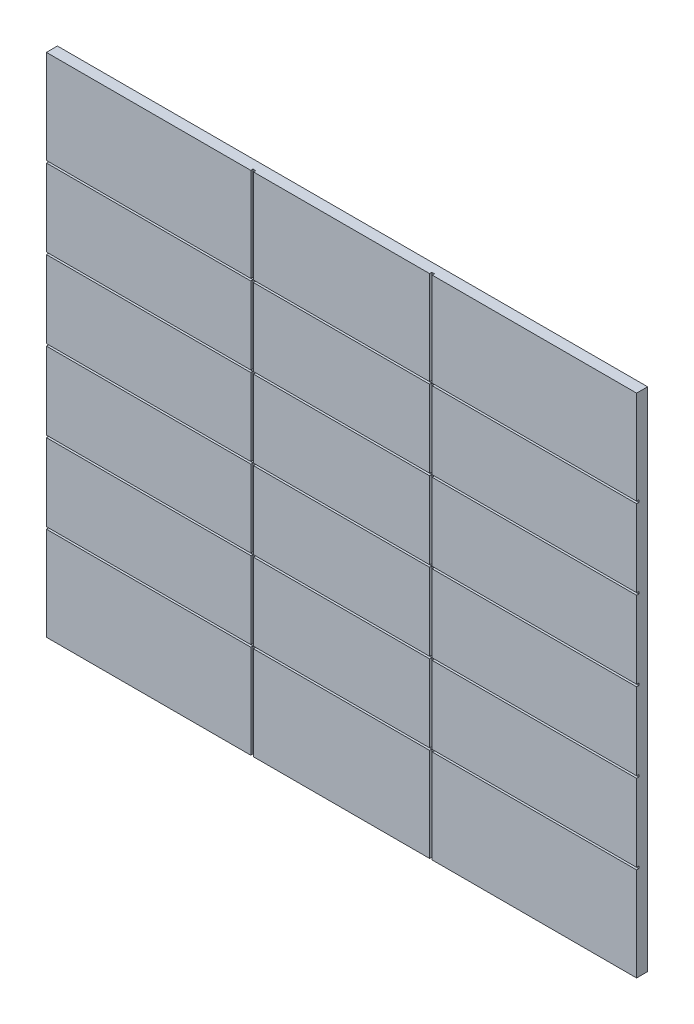
SolidWorks part; units mm, degrees
ref_plane "Front Plane" through (0, 0, 0) normal (0, 0, 1) x (1, 0, 0)
ref_plane "Top Plane" through (0, 0, 0) normal (0, 1, 0) x (1, 0, 0)
ref_plane "Right Plane" through (0, 0, 0) normal (1, 0, 0) x (0, 0, -1)
sketch "Sketch1" plane through (0, 0, 0) normal (0, 0, 1) x (1, 0, 0)
  line L1 (-670, 575) -> (670, 575)
  line L2 (-670, 575) -> (-670, -575)
  line L3 (-670, -575) -> (670, -575)
  line L4 (670, 575) -> (670, -575)
  line L5 (-670, 575) -> (670, -575) construction
  line L6 (-670, -575) -> (670, 575) construction
  point P0 (0, 0)
  dimension "D1" = 1340
  dimension "D2" = 1150
extrude "Boss-Extrude1" add sketch "Sketch1" along normal blind 25
sketch "Sketch2" plane through (0, 0, 25) normal (0, 0, 1) x (1, 0, 0)
  line L1 (-689.8522, 2.5) -> (689.8522, 2.5)
  line L2 (-689.8522, 2.5) -> (-689.8522, -2.5)
  line L3 (-689.8522, -2.5) -> (689.8522, -2.5)
  line L4 (689.8522, 2.5) -> (689.8522, -2.5)
  line L5 (-689.8522, 2.5) -> (689.8522, -2.5) construction
  line L6 (-689.8522, -2.5) -> (689.8522, 2.5) construction
  point P0 (0, 0)
  dimension "D1" = 5
extrude "Cut-Extrude1" cut sketch "Sketch2" against normal blind 5
sketch "Sketch3" plane through (0, 0, 25) normal (0, 0, 1) x (1, 0, 0)
  line L0 (0, 0) -> (0, 486.5607) construction
  line L1 (200, 577.0918) -> (206, 577.0918)
  line L2 (200, 577.0918) -> (200, -578.2429)
  line L3 (200, -578.2429) -> (206, -578.2429)
  line L4 (206, 577.0918) -> (206, -578.2429)
  line L5 (200, 577.0918) -> (206, -578.2429) construction
  line L6 (200, -578.2429) -> (206, 577.0918) construction
  line L7 (-200, 577.0918) -> (-206, 577.0918)
  line L8 (-200, -578.2429) -> (-206, -578.2429)
  line L9 (-206, 577.0918) -> (-206, -578.2429)
  line L10 (-200, 577.0918) -> (-200, -578.2429)
  point P0 (203, -0.5755)
  dimension "D1" = 6
  dimension "D2" = 200
extrude "Cut-Extrude2" cut sketch "Sketch3" against normal blind 5
pattern_linear "LPattern1" count 3 spacing 180 along (0, -1, 0) count 3 spacing 180 along (0, 1, 0) seed only of "Cut-Extrude1"
sketch "Sketch4" plane through (-49.5237, -434, -370.2813) normal (0, -1, 0) x (0.9899, 0, -0.1414)
  line L0 (362.9416, 425.8894) -> (367.1842, 396.1909)
  line L1 (-666.6059, 278.8112) -> (659.9264, 468.3158) construction
  line L2 (656.3909, 493.0646) -> (659.9264, 468.3158) construction
  dimension "D1" = 30
  dimension "D2" = 300
sweep "Sweep1" add path "Sketch4" circular profile diameter 10 parameters "D3"=10
sketch "Sketch13" plane through (0, 0, -30) normal (0, 0, -1) x (-1, 0, 0)
  circle A0 centre (-370, -434) radius 1.5
  dimension "D1" = 3
extrude "Cut-Extrude3" cut sketch "Sketch13" against normal blind 10
